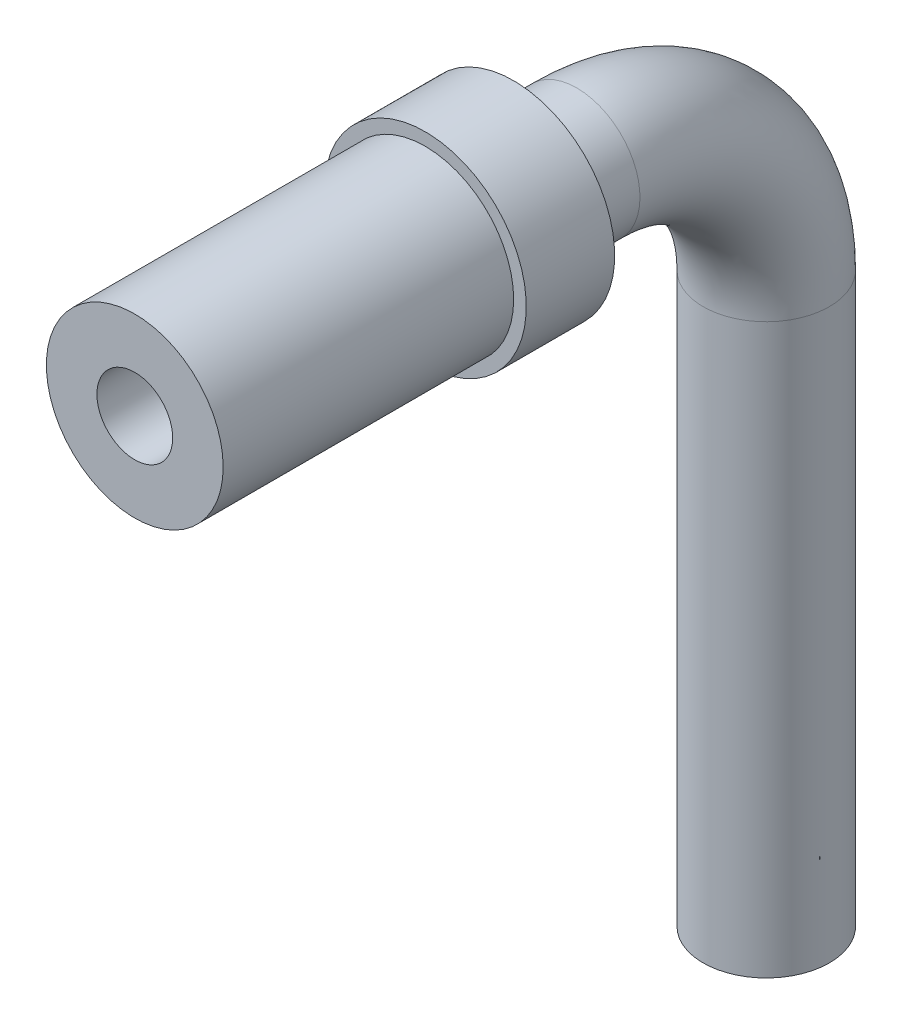
from build123d import *

# Parameters (mm, degrees)
SKETCH2_R           = 5
SKETCH2_R_2         = 3
BOSS_EXTRUDE1_START = -30
SKETCH3_R           = 7
SKETCH3_R_2         = 5
BOSS_EXTRUDE1_DEPTH = 30
SKETCH4_R           = 8
SKETCH4_R_2         = 7
BOSS_EXTRUDE2_DEPTH = 7


with BuildPart() as part:
    # Sweep1: sweep along a path in Sketch1
    with BuildLine(Plane(origin=(0, 0, 0), x_dir=(0, 0, -1), z_dir=(1, 0, 0))) as sweep1_path:
        Line((0, 0), (35, 0))
        ThreePointArc((35, 0), (45.606601718, -4.393398282), (50, -15))
        Line((50, -15), (50, -60))
    # Sketch2 → Sweep1 (sweep)
    with BuildSketch(Plane.XY):
        Circle(SKETCH2_R)
        Circle(SKETCH2_R_2, mode=Mode.SUBTRACT)
    sweep(path=sweep1_path.line)

    # Sketch3 → Boss-Extrude1 (add)
    with BuildSketch(Plane.XY.offset(BOSS_EXTRUDE1_START)):
        Circle(SKETCH3_R)
        with Locations(Location((0, 0, 0), (0, 0, 90))):
            Circle(SKETCH3_R_2, mode=Mode.SUBTRACT)
    extrude(amount=BOSS_EXTRUDE1_DEPTH)

    # Sketch4 → Boss-Extrude2 (add)
    with BuildSketch(Plane(origin=(0, 0, -30), x_dir=(-1, 0, 0), z_dir=(0, 0, -1))):
        Circle(SKETCH4_R)
        with Locations(Location((0, 0, 0), (0, 0, 180))):
            Circle(SKETCH4_R_2, mode=Mode.SUBTRACT)
    extrude(amount=-BOSS_EXTRUDE2_DEPTH)


solid = part.part
